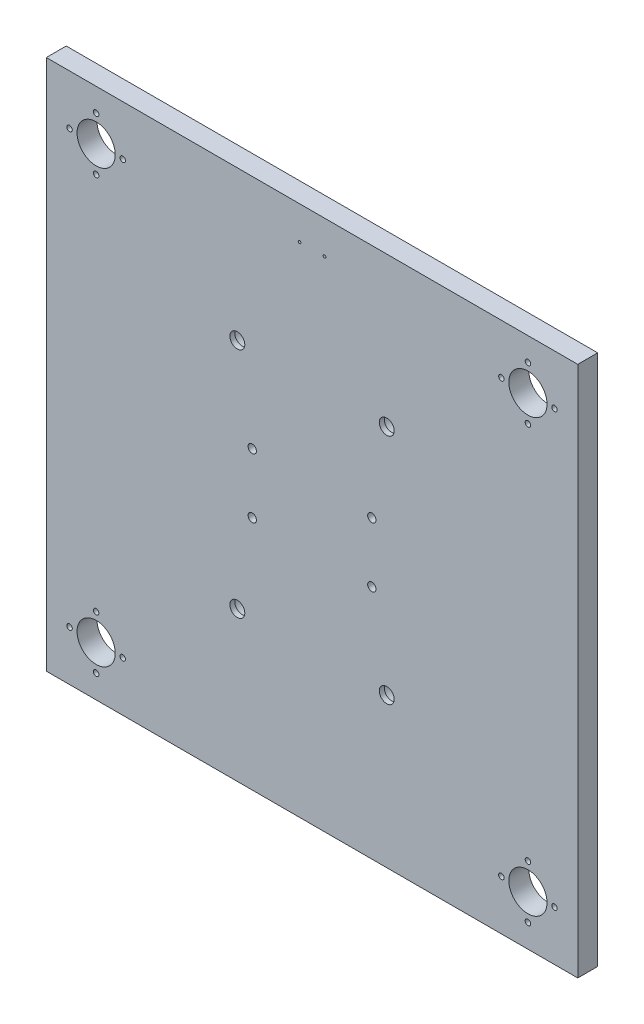
from build123d import *

# Parameters (mm, degrees)
SKETCH_1_W                = 320
SKETCH_1_H                = 320
SKETCH_1_R                = 11.5
EXTRUDE_1_DEPTH           = 6
HOLE_WIZARD_M6_1_D        = 5
HOLE_WIZARD_1_D           = 9
HOLE_WIZARD_1_CBORE_D     = 15
HOLE_WIZARD_1_CBORE_DEPTH = 9
HOLE_WIZARD_M4_2_D        = 3.3
MIRROR_2_COPY_1_D         = 3.3
HOLE_WIZARD_M4_1_D        = 3.3
HOLE_WIZARD_M4_1_DEPTH    = 11.5
HOLE_WIZARD_M4_1_TIP      = 0.991420021


with BuildPart() as part:
    # 草图1 → 凸台-拉伸1 (new, symmetric)
    with BuildSketch(Plane.XY):
        Rectangle(SKETCH_1_W, SKETCH_1_H)
        with Locations((-130, 130)):
            Circle(SKETCH_1_R, mode=Mode.SUBTRACT)
        with Locations((130, 130)):
            Circle(SKETCH_1_R, mode=Mode.SUBTRACT)
        with Locations((130, -130)):
            Circle(SKETCH_1_R, mode=Mode.SUBTRACT)
        with Locations((-130, -130)):
            Circle(SKETCH_1_R, mode=Mode.SUBTRACT)
    extrude(amount=EXTRUDE_1_DEPTH, both=True)

    # M6 螺纹孔1 (through all)
    with Locations(Plane(origin=(0, 0, -6), x_dir=(-1, 0, 0), z_dir=(0, 0, -1))):
        with Locations((-36, 18), (-36, -18), (36, -18), (36, 18)):
            Hole(HOLE_WIZARD_M6_1_D / 2)

    # 打孔尺寸(%根据)内六角圆柱头螺钉的类型1 (through all)
    with Locations(Plane(origin=(0, 0, -6), x_dir=(-1, 0, 0), z_dir=(0, 0, -1))):
        with Locations((-45, 70), (45, 70), (45, -70), (-45, -70)):
            CounterBoreHole(HOLE_WIZARD_1_D / 2, HOLE_WIZARD_1_CBORE_D / 2, HOLE_WIZARD_1_CBORE_DEPTH)

    # M4 螺纹孔2 (through all)
    with Locations(Plane.XY.offset(6)):
        with Locations((-130, 146), (-114, 130), (-130, 114), (-146, 130)):
            hole_wizard_m4_2 = Hole(HOLE_WIZARD_M4_2_D / 2)

    # 镜向1: M4 螺纹孔2 across plane
    add(hole_wizard_m4_2.mirror(Plane.ZX), mode=Mode.SUBTRACT)

    # 镜向2: M4 螺纹孔2 across plane
    add(hole_wizard_m4_2.mirror(Plane(origin=(0, 0, 0), x_dir=(0, 0, 1), z_dir=(1, 0, 0))), mode=Mode.SUBTRACT)

    # 镜向2 copy 1 (through all)
    with Locations(Plane(origin=(0, 0, 6), x_dir=(-1, 0, 0), z_dir=(0, 0, 1))):
        with Locations((-130, 146), (-114, 130), (-130, 114), (-146, 130)):
            Hole(MIRROR_2_COPY_1_D / 2)

    # M4 螺纹孔1
    with Locations(Plane(origin=(0, 0, -6), x_dir=(-1, 0, 0), z_dir=(0, 0, -1))):
        with Locations((-7.5, 140), (7.5, 140)):
            Hole(HOLE_WIZARD_M4_1_D / 2, depth=HOLE_WIZARD_M4_1_DEPTH)
            with Locations((0, 0, -(HOLE_WIZARD_M4_1_DEPTH + HOLE_WIZARD_M4_1_TIP / 2))):  # 118° drill point
                Cone(0, HOLE_WIZARD_M4_1_D / 2, HOLE_WIZARD_M4_1_TIP, mode=Mode.SUBTRACT)


solid = part.part
